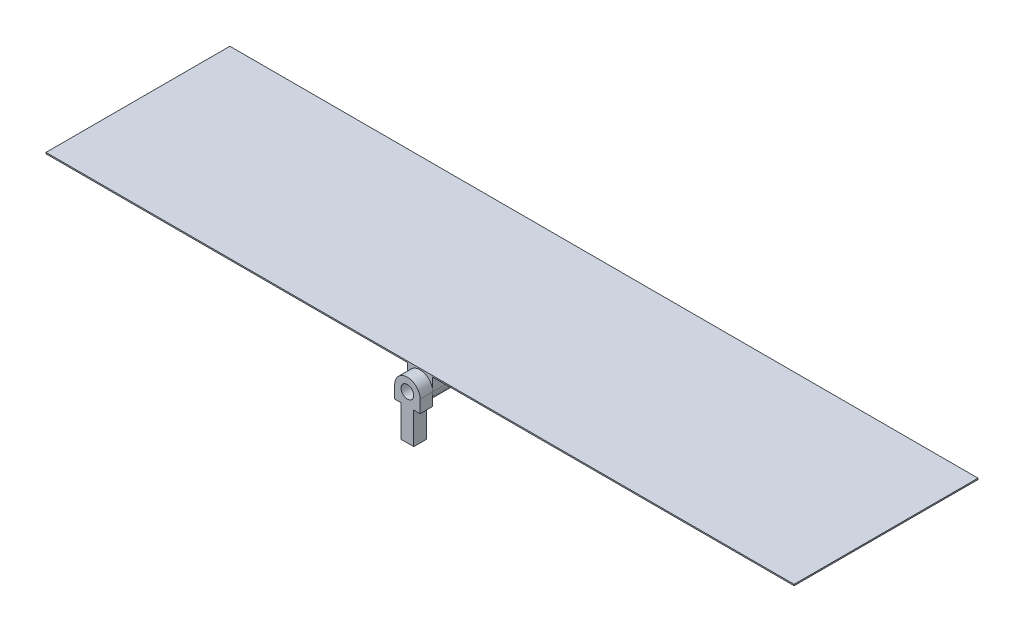
from build123d import *

# Parameters (mm, degrees)
SKETCH_1_R      = 5
EXTRUDE_1_DEPTH = 72.5
SKETCH_2_W      = 590
SKETCH_2_H      = 145
EXTRUDE_2_DEPTH = 1
EXTRUDE_3_DEPTH = 5
SKETCH_5_R      = 5
EXTRUDE_4_DEPTH = 10


with BuildPart() as part:
    # 草图1 → 凸台-拉伸1 (new, symmetric)
    with BuildSketch(Plane.XY):
        with BuildLine():
            Line((-10, 0), (-10, 10))
            Line((-10, 10), (10, 10))
            Line((10, 10), (10, 0))
            ThreePointArc((10, 0), (0, -10), (-10, 0))
        make_face()
        Circle(SKETCH_1_R, mode=Mode.SUBTRACT)
    extrude(amount=EXTRUDE_1_DEPTH, both=True)



with BuildPart() as body_2:
    # 草图2 → 凸台-拉伸2 (new body)
    with BuildSketch(Plane(origin=(0, 10, 0), x_dir=(1, 0, 0), z_dir=(0, 1, 0))):
        Rectangle(SKETCH_2_W, SKETCH_2_H)
    extrude(amount=EXTRUDE_2_DEPTH)


with BuildPart() as part_1:
    add(part.part)

    add(body_2.part)  # 凸台-拉伸3 merges body 2
    # 草图4 → 凸台-拉伸3 (add, symmetric)
    with BuildSketch(Plane.XY):
        with BuildLine():
            Line((-10, 10), (-250, 10))
            Line((-250, 10), (-250, 5))
            Line((-250, 5), (-0.599640103, -9.982005397))
            ThreePointArc((-0.599640103, -9.982005397), (-7.279986299, -6.85578584), (-10, 0))
            Line((-10, 0), (-10, 10))
        make_face()
        with BuildLine():
            Line((10, 10), (249.997916658, 11))
            Line((249.997916658, 11), (249.997916658, 6))
            Line((249.997916658, 6), (0.639514993, -9.979530078))
            ThreePointArc((0.639514993, -9.979530078), (7.293666771, -6.84122979), (10, 0))
            Line((10, 0), (10, 10))
        make_face()
    extrude(amount=EXTRUDE_3_DEPTH, both=True)

    # 草图5 → 凸台-拉伸4 (add)
    with BuildSketch(Plane.XY.offset(72.5)):
        with BuildLine():
            Line((-10, 0), (-10, -10))
            Line((-10, -10), (-5, -10))
            Line((-5, -10), (-5, -25))
            Line((-5, -25), (-5, -35))
            Line((-5, -35), (5, -35))
            Line((5, -35), (5, -25))
            Line((5, -25), (5, -10))
            Line((5, -10), (10, -10))
            Line((10, -10), (10, 0))
            ThreePointArc((10, 0), (0, 10), (-10, 0))
        make_face()
        Circle(SKETCH_5_R, mode=Mode.SUBTRACT)
    extrude(amount=EXTRUDE_4_DEPTH)


solid = part_1.part
